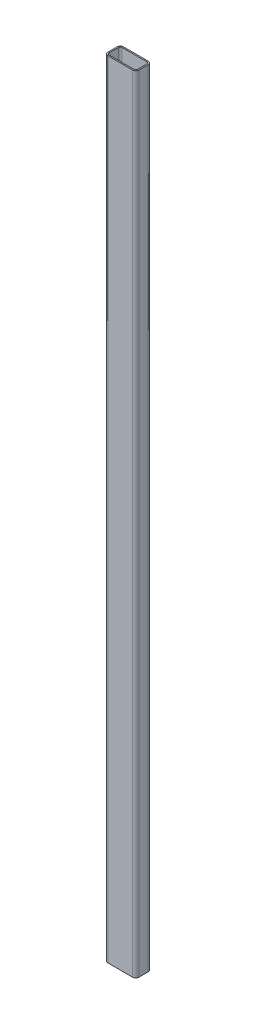
SolidWorks part; units mm, degrees
ref_plane "Front Plane" through (0, 0, 0) normal (0, 0, 1) x (1, 0, 0)
ref_plane "Top Plane" through (0, 0, 0) normal (0, 1, 0) x (1, 0, 0)
ref_plane "Right Plane" through (0, 0, 0) normal (1, 0, 0) x (0, 0, -1)
other "Configuration Table"
sketch "Sketch1" plane through (0, 0, 0) normal (0, 1, 0) x (1, 0, 0)
  line L1 (-40, 25) -> (40, 25)
  line L2 (-50, 15) -> (-50, -15)
  line L3 (-40, -25) -> (40, -25)
  line L4 (50, 15) -> (50, -15)
  line L5 (-50, 25) -> (50, -25) construction
  line L6 (-50, -25) -> (50, 25) construction
  arc A0 (40, 25) -> (50, 15) centre (40, 15) cw
  arc A1 (40, -25) -> (50, -15) centre (40, -15) ccw
  arc A2 (-50, -15) -> (-40, -25) centre (-40, -15) ccw
  arc A3 (-40, 25) -> (-50, 15) centre (-40, 15) ccw
  point P0 (0, 0)
  dimension "D3" = 10
  dimension "D1" = 100
  dimension "D2" = 50
extrude "Extrude-Thin1" add sketch "Sketch1" along normal mid plane 2530 thin
